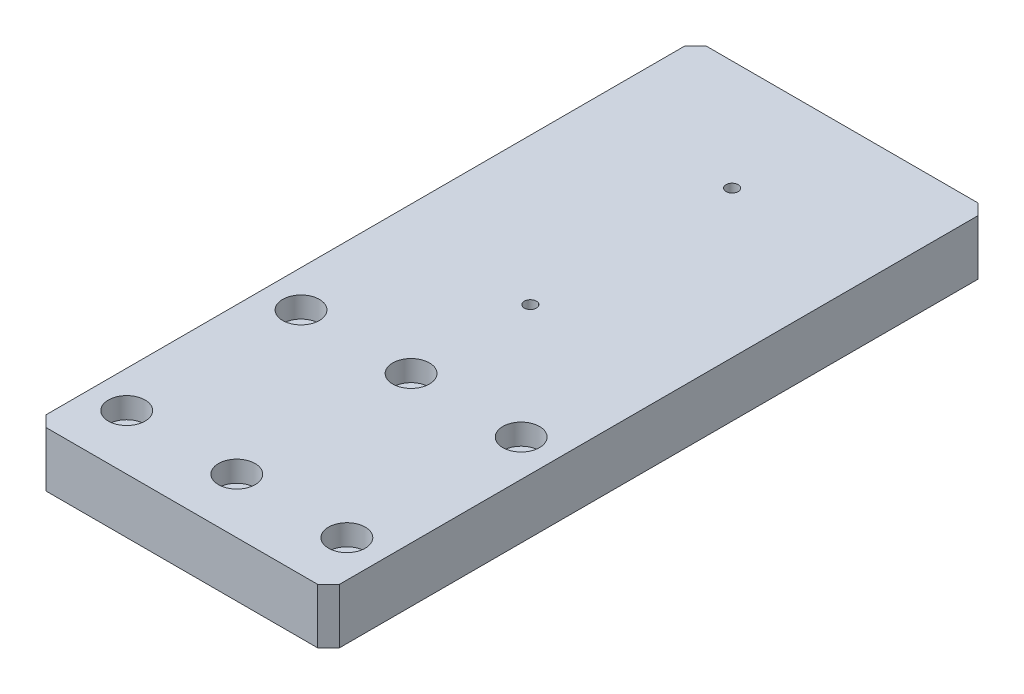
from build123d import *

# Parameters (mm, degrees)
SKETCH_1_W                = 80
SKETCH_1_H                = 180
EXTRUDE_1_DEPTH           = 15
CHAMFER_1_SIZE            = 3
HOLE_WIZARD_M4_1_D        = 3.3
HOLE_WIZARD_M4_1_DEPTH    = 20
HOLE_WIZARD_M4_1_TIP      = 0.991420021
HOLE_WIZARD_1_D           = 5.5
HOLE_WIZARD_1_DEPTH       = 20
HOLE_WIZARD_1_CBORE_D     = 10
HOLE_WIZARD_1_CBORE_DEPTH = 5.7
HOLE_WIZARD_1_TIP         = 1.652366702
HOLE_WIZARD_2_D           = 5.5
HOLE_WIZARD_2_DEPTH       = 15
HOLE_WIZARD_2_CBORE_D     = 10
HOLE_WIZARD_2_CBORE_DEPTH = 5.7
HOLE_WIZARD_2_TIP         = 1.652366702


with BuildPart() as part:
    # 草图1 → 凸台-拉伸1 (new body)
    with BuildSketch(Plane(origin=(0, 0, 0), x_dir=(1, 0, 0), z_dir=(0, 1, 0))):
        Rectangle(SKETCH_1_W, SKETCH_1_H)
    extrude(amount=EXTRUDE_1_DEPTH)

    # 倒角1
    chamfer_1_edges = [part.edges().sort_by_distance(p)[0] for p in [
        (40, 7.5, 90),
        (-40, 7.5, 90),
        (-40, 7.5, -90),
        (40, 7.5, -90),
    ]]
    chamfer(chamfer_1_edges, length=CHAMFER_1_SIZE)

    # M4 螺纹孔1
    with Locations(Plane(origin=(0, 15, 0), x_dir=(1, 0, 0), z_dir=(0, 1, 0))):
        with Locations((0, 60), (0, 5)):
            Hole(HOLE_WIZARD_M4_1_D / 2, depth=HOLE_WIZARD_M4_1_DEPTH)
            with Locations((0, 0, -(HOLE_WIZARD_M4_1_DEPTH + HOLE_WIZARD_M4_1_TIP / 2))):  # 118° drill point
                Cone(0, HOLE_WIZARD_M4_1_D / 2, HOLE_WIZARD_M4_1_TIP, mode=Mode.SUBTRACT)

    # 打孔尺寸(%根据)内六角圆柱头螺钉的类型1
    with Locations(Plane(origin=(0, 15, 0), x_dir=(1, 0, 0), z_dir=(0, 1, 0))):
        with Locations((-30, -27.5), (0, -27.5), (30, -27.5)):
            CounterBoreHole(HOLE_WIZARD_1_D / 2, HOLE_WIZARD_1_CBORE_D / 2, HOLE_WIZARD_1_CBORE_DEPTH, depth=HOLE_WIZARD_1_DEPTH)
            with Locations((0, 0, -(HOLE_WIZARD_1_DEPTH + HOLE_WIZARD_1_TIP / 2))):  # 118° drill point
                Cone(0, HOLE_WIZARD_1_D / 2, HOLE_WIZARD_1_TIP, mode=Mode.SUBTRACT)

    # 打孔尺寸(%根据)内六角圆柱头螺钉的类型2
    with Locations(Plane(origin=(0, 15, 0), x_dir=(1, 0, 0), z_dir=(0, 1, 0))):
        with Locations((-30, -75), (0, -75), (30, -75)):
            CounterBoreHole(HOLE_WIZARD_2_D / 2, HOLE_WIZARD_2_CBORE_D / 2, HOLE_WIZARD_2_CBORE_DEPTH, depth=HOLE_WIZARD_2_DEPTH)
            with Locations((0, 0, -(HOLE_WIZARD_2_DEPTH + HOLE_WIZARD_2_TIP / 2))):  # 118° drill point
                Cone(0, HOLE_WIZARD_2_D / 2, HOLE_WIZARD_2_TIP, mode=Mode.SUBTRACT)


solid = part.part
